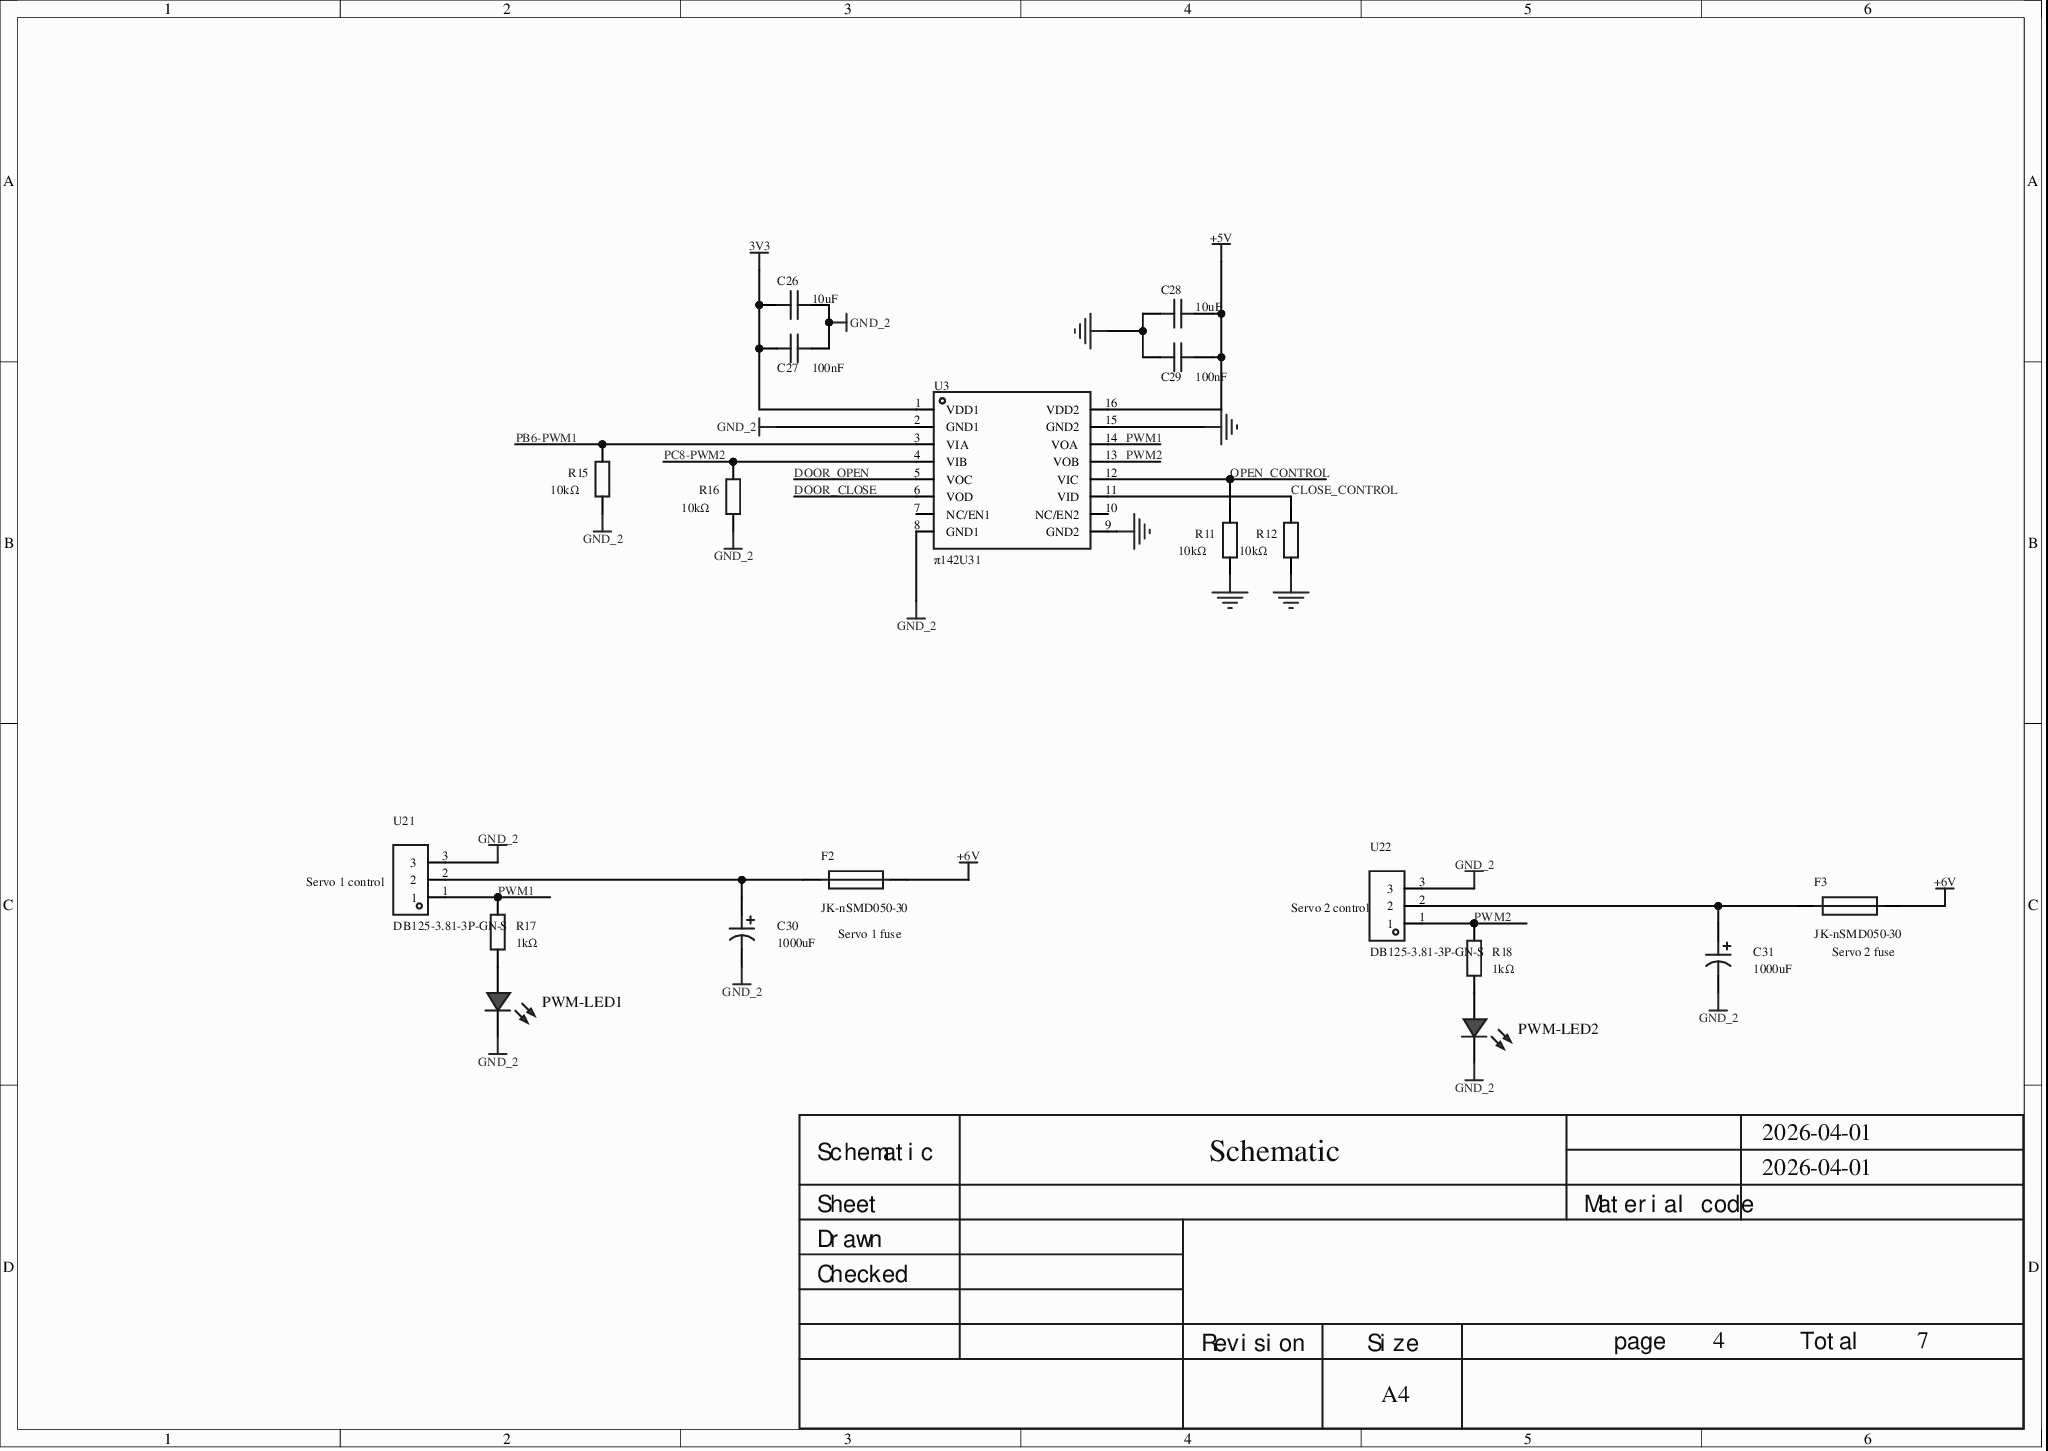
[diagram p0: MISC49876-5.schdoc]
# Altium project MISC49876-2.PrjPcb (part 2 of 2)
## Sheet MISC49876-5.schdoc (continued)
### Nets (continued)
CLOSE_CONTROL: R12.2 U3.11(VID)
DOOR_CLOSE: U3.6(VOD)
DOOR_OPEN: U3.5(VOC)
OPEN_CONTROL: R11.2 U3.12(VIC)
PB6-PWM1: R15.2 U3.3(VIA)
PC8-PWM2: R16.2 U3.4(VIB)
PWM1: R17.2 U3.14(VOA) U21.1
PWM2: R18.2 U3.13(VOB) U22.1
NetC30_1: C30.1 F2.1 U21.2
NetC31_1: C31.1 F3.1 U22.2
NetPWM-LED1_2: PWM-LED1.2(A) R17.1
NetPWM-LED2_2: PWM-LED2.2(A) R18.1

Not connected (* = marked no-connect by the designer): U3 7(NC/EN1) 10(NC/EN2)

### Notes on the sheet
- (near U21) Servo 1 control
- (near F2) Servo 1 fuse
- (near U22) Servo 2 control
- (near F3) Servo 2 fuse
- 2026-04-01
- Schematic
- Sheet
- Material code
- Checked
- Drawn
- Revision
- Size
- A4
- page
- 4
- Total
- 7

### Library data of the parts
C26 = GRM21BR61H106KE43L: Capacitance: 10uF; tolerance: ±10%; rated voltage: 50V; dielectric (temp. coefficient): X5R;; Manufacturer: muRata(村田); 3D Model: 1ba041120af144c991958decab20d241; 3D Model Transform: 78.74,51.181,0,0,0,0,0,0.0005,0; AddInBom: yes; ModelName: C0805_L2.0-W1.3-H1.3; Symbol: GRM21BR61H106KE43L; Device: GRM21BR61H106KE43L; LCSC Part Name: 10uF ±10% 50V; Supplier Footprint: 0805; Datasheet: https://atta.szlcsc.com/upload/public/pdf/source/20230811/95AAE0C9AF55EDC31B7A4D8B733F534E.pdf; Tolerance: ±10%; Voltage Rated: 50V; Temperature Coefficient: X5R; Supplier: LCSC; Supplier Part: C440198; Manufacturer Part: GRM21BR61H106KE43L; Value: 10uF; JLCPCB Part Class: Basic Part; ConvertToPcb: yes; FootprintName: C0805
C27 = CC0603KRX7R9BB104: Capacitance: 100nF; tolerance: ±10%; rated voltage: 50V; dielectric (temp. coefficient): X7R;; Manufacturer: YAGEO(国巨); Symbol: 0.1u; Add into BOM: yes; 3D Model: ac125912035d415993ca9572d50418b1; 3D Model Transform: 62.992,31.496,0,0,0,0,0,0,0; ModelName: C0603_L1.6-W0.8-H0.8; Device: CC0603KRX7R9BB104; Convert to PCB: yes; Origin Footprint: C0603; Supplier Part: C14663; Supplier: LCSC; Manufacturer Part: CC0603KRX7R9BB104; JLCPCB Part Class: Basic Part; LCSC Part Name: 100nF ±10% 50V; Supplier Footprint: 0603; Datasheet: https://atta.szlcsc.com/upload/public/pdf/source/20180910/C282072_33301C7F631E79921B82A8DAC6BCC5B3.pdf; Value: 100nF; Tolerance: ±10%; Voltage Rated: 50V; Temperature Coefficient: X7R; FootprintName: C0603
C28 = GRM21BR61H106KE43L: Capacitance: 10uF; tolerance: ±10%; rated voltage: 50V; dielectric (temp. coefficient): X5R;; Manufacturer: muRata(村田); AddInBom: yes; ModelId: 1ba041120af144c991958decab20d241; ModelName: C0805_L2.0-W1.3-H1.3; ModelTransform: 78.74,51.181,0,0,0,0,0,0.0005,0; Symbol: GRM21BR61H106KE43L; Device: GRM21BR61H106KE43L; Supplier: LCSC; Supplier Part: C440198; Manufacturer Part: GRM21BR61H106KE43L; Value: 10uF; JLCPCB Part Class: Basic Part; LCSC Part Name: 10uF ±10% 50V; Supplier Footprint: 0805; Datasheet: https://atta.szlcsc.com/upload/public/pdf/source/20230811/95AAE0C9AF55EDC31B7A4D8B733F534E.pdf; ConvertToPcb: yes; FootprintName: C0805; Tolerance: ±10%; Voltage Rated: 50V; Temperature Coefficient: X5R
C29 = CC0603KRX7R9BB104: as C6 on sheet MISC49876-3; Origin Footprint: C0603; Device: CC0603KRX7R9BB104; Supplier Part: C14663; Supplier: LCSC; Manufacturer Part: CC0603KRX7R9BB104; Add into BOM: yes; JLCPCB Part Class: Basic Part; LCSC Part Name: 100nF ±10% 50V; Supplier Footprint: 0603; Datasheet: https://atta.szlcsc.com/upload/public/pdf/source/20180910/C282072_33301C7F631E79921B82A8DAC6BCC5B3.pdf; FootprintName: C0603; Value: 100nF; Tolerance: ±10%; Voltage Rated: 50V; Temperature Coefficient: X7R
C30 C31 = SPZ0JM102E10C35RAXXX: Capacitance: 1000uF; tolerance: ±20%; rated voltage: 6.3V;; Manufacturer: AISHI(艾华集团); AddInBom: yes; ModelId: 983aa343eddc42b59ebb10541a88166e; ModelTransform: 247.99486,248.229,0,90,0,0,0,0,-196.85; Symbol: SPZ0JM102E10C35RAXXX; Device: SPZ0JM102E10C35RAXXX; LCSC Part Name: 1000uF ±20% 6.3V; SupplierPart: C5349927; ManufacturerPart: SPZ0JM102E10C35RAXXX; Supplier Footprint: 插件,D6.3xL10mm; JLCPCB Part Class: Extended Part; Datasheet: https://atta.szlcsc.com/upload/public/pdf/source/20230106/1004933EB9CF55C39AD0630773DFF44F.pdf; Supplier: LCSC; ConvertToPcb: yes; FootprintName: CAP-TH_BD6.3-P2.50-D0.5-FD; ModelName: CAP-TH_BD6.3-P2.50-D0.5-FD; Value: 1000uF; Tolerance: ±20%; Rated Voltage: 6.3V
F2 F3 = JK-nSMD050-30: Max voltage: 30V; max current: 100A; hold current: 500mA; trip current: 1A;; Manufacturer: JK(金科); Symbol: JK-NSMD050-30V; AddInBom: yes; ModelId: f1628daad26847a79b887277a2bc8541; ModelName: F1206_L3.2-W1.7-H0.6; ModelTransform: 125.984,66.929,0,0,0,0,0,0,0; Power Dissipation: 600mW; Resistance - Initial (Ri) (Min): 150mΩ; Resistance - Post Trip (R1) (Max): 300mΩ; Maximum Time to Trip: 100ms; Device: JK-nSMD050-30; Supplier: LCSC; Supplier Part: C720075; Manufacturer Part: JK-nSMD050-30; JLCPCB Part Class: Extended library; LCSC Part Name: 30V 500mA 1206自恢复; Supplier Footprint: 1206; Datasheet: https://atta.szlcsc.com/upload/public/pdf/source/20200810/C720075_06AF2D4541537091880CC35F0EFB49F8.pdf; ConvertToPcb: yes; FootprintName: F1206; Operating Voltage (Max): 30V; Current Rating (Max): 100A; Hold Current: 500mA; Trip Current: 1A; Operating Temperature: -40℃~+85℃
PWM-LED1 PWM-LED2 = LED_0603-R: Symbol: LED_R; Convert to PCB: yes; 3D Model: dd8257b0d61a4cd7b68939a056e08095; 3D Model Transform: 58.72,29.4,22.03,0,0,0,0,0,0; ModelName: LED-0603_R; Device: LED_0603-R; Add into BOM: yes; Supplier Footprint: 0603; FootprintName: LED_0603
R11 R12 R15 R16 = 0603WAF3301T5E: Resistor type: thick film resistor; resistance: 3.3kΩ; tolerance: ±1%; power: 100mW; max working voltage: 75V; temp. coefficient: ±100ppm/℃;; Manufacturer: UNI-ROYAL(厚声); 3D Model: fc143cca1e79419f9cd78b61e9279f08; 3D Model Transform: 31.8897,63.7794,0,90,0,0,0,0,0; AddInBom: yes; Symbol: 0603WAF3301T5E; Device: 0603WAF3301T5E; Value: 10kΩ; LCSC Part Name: 3.3kΩ ±1% 100mW 厚膜电阻; Supplier Footprint: 0603; Datasheet: https://atta.szlcsc.com/upload/public/pdf/source/20200306/C422600_1E6D84923E4A46A82E41ADD87F860B5C.pdf; Type: Thick film resistor; Tolerance: ±1%; Power(Watts): 100mW; Overload Voltage (Max): 75V; Temperature Coefficient: ±100ppm/℃; Operating Temperature Range: -55℃~+155℃; Supplier: LCSC; Manufacturer Part: 0603WAF3301T5E; JLCPCB Part Class: Basic library; ConvertToPcb: yes; FootprintName: R0603; ModelName: R0603
R17 R18 = 0603WAF1001T5E: Resistance: 1kΩ; tolerance: ±1%; power: 100mW; temp. coefficient: ±100ppm/℃; resistor type: thick film resistor;; Manufacturer: UNI-ROYAL(厚声); Symbol: 0603waf1301t5e; AddInBom: yes; ModelId: fc143cca1e79419f9cd78b61e9279f08; ModelTransform: 31.8897,63.7794,0,90,0,0,0,0,0; Overload Voltage (Max): 75V; Device: 0603WAF1001T5E; Supplier: LCSC; Manufacturer Part: 0603WAF1001T5E; Supplier Part: C21190; Value: 1kΩ; JLCPCB Part Class: Basic Part; LCSC Part Name: 1kΩ ±1% 100mW 厚膜电阻; Supplier Footprint: 0603; Datasheet: https://atta.szlcsc.com/upload/public/pdf/source/20200306/C422600_1E6D84923E4A46A82E41ADD87F860B5C.pdf; ConvertToPcb: yes; FootprintName: R0603; ModelName: R0603; Tolerance: ±1%; Power(Watts): 100mW; Temperature Coefficient: ±100ppm/℃; Type: Thick film resistor; Operating Temperature Range: -55℃~+155℃
U3 = π142U31: 通过使用成熟的标准半导体CMOS技术和iDivider技术，这些隔离组件提供了出色的性能特性和可靠性，优于光耦设备和其他集成隔离器等替代产品。智能分压器技术（iDivider技术）是一种新一代数字隔离器技术，它利用电容分压器原理直接跨隔离器电容传输电压信号，无需信号调制和解调。隔离器数据通道独立，有多种配置可供选择，耐压额定值为1.5kV rms至6.0kV rms，数据速率从直流到600Mbps。设备两侧的电源电压范围为3.0V至5.5V，可与低电压系统兼容，并能在隔离屏障上实现电压转换功能。当未施加输; Manufacturer: 2Pai Semi(荣湃); AddInBom: yes; ModelId: c21ec766ec2643efb3352f8441994f4e0819f05c4eef4c71ace90d822a990e87; ModelName: SOIC-16_L9.9-W3.9-H1.8-LS6.0-P1.27; ModelTransform: 389.763,236.454,0,0,0,0,0,0,0; Number of Forward Channels: 2; Data Rate(Max): 150Kbps; Isolation Voltage(Vrms): 3000; CMTI(kV/us): 150kV/us; Propagation Delay(tpd): 4.5us; Voltage - Supply(VCCA): 3V~5.5V; Symbol: π142U31; Device: π142U31; LCSC Part Name: 增强ESD 3.0 kVrms/6.0 kVrms 150Kbps四通道数字隔离器; SupplierPart: C471603; ManufacturerPart: π142U31; Supplier Footprint: SOIC-16; JLCPCB Part Class: Extended Part; Datasheet: https://item.szlcsc.com/datasheet/%25CF%2580142U31/478045.html; Supplier: LCSC; ConvertToPcb: yes; FootprintName: SOIC-16_L9.9-W3.9-P1.27-LS6.0-BL; Number of Reverse Channels: 2; Default Output: -; Features: Multi-voltage-domain interface; fail-safe output; Voltage - Supply(VCCB): 3V~5.5V; Operating Temperature: -40℃~+125℃
U21 U22 = DB125-3.81-3P-GN-S: 结构:1x3P;间距:3.81mm;颜色:绿色;安装方式:直插;额定电流:10A;额定电压:300V;排数:1;线规 - AWG:16~26;线规 - 平方毫米:0.5~1;每排PIN数:3;工作温度范围:-40℃~+105℃;; Manufacturer: DORABO(地博电气); AddInBom: yes; ModelId: eb9d9db6d88745c4b1f598d16985b52f; ModelName: CONN-TH_DB3.81-LI-3P-125; ModelTransform: 469.6739,291.338,0,0,0,0,-11.811,11.811,-157.48; Structure: 1x3P; Pitch: 3.81mm; Current Rating (Max): 10A; Voltage Rating (Max): 300V; Wire Gauge - AWG: 16~26; Wire Gauge - mm2: 0.5~1; Number of PINs Per Row: 3; Symbol: DB125-3.81-3P; Device: DB125-3.81-3P-GN-S; LCSC Part Name: 3.81mm 1x3P 排数:1 每排P数:3 直插; SupplierPart: C395879; ManufacturerPart: DB125-3.81-3P-GN-S; Supplier Footprint: 插件,P=3.81mm; JLCPCB Part Class: Extended library; Datasheet: https://atta.szlcsc.com/upload/public/pdf/source/20220823/CB89165D0F406880B925A92BEEA3FB50.pdf; Supplier: LCSC; ConvertToPcb: yes; FootprintName: CONN-TH_3P-P3.81_L7.4-W11.4; Color: Green; Mounting Style: Through-hole; Number of Pins: 3P; Number of Rows: 1; Operating Temperature Range: -40℃~+105℃

## Sheet MISC49876-4.schdoc
size 297 x 210 mm; Version: V1.0; @Project Name: MISC49876; @Page Count: 7; @Update Date: 2026-04-01; @Create Date: 2026-04-01; @Schematic Name: MISC49876; @Page No: 1; @Board Name: MISC49876; @Create Time: 07:49:54; @Update Time: 15:55:16
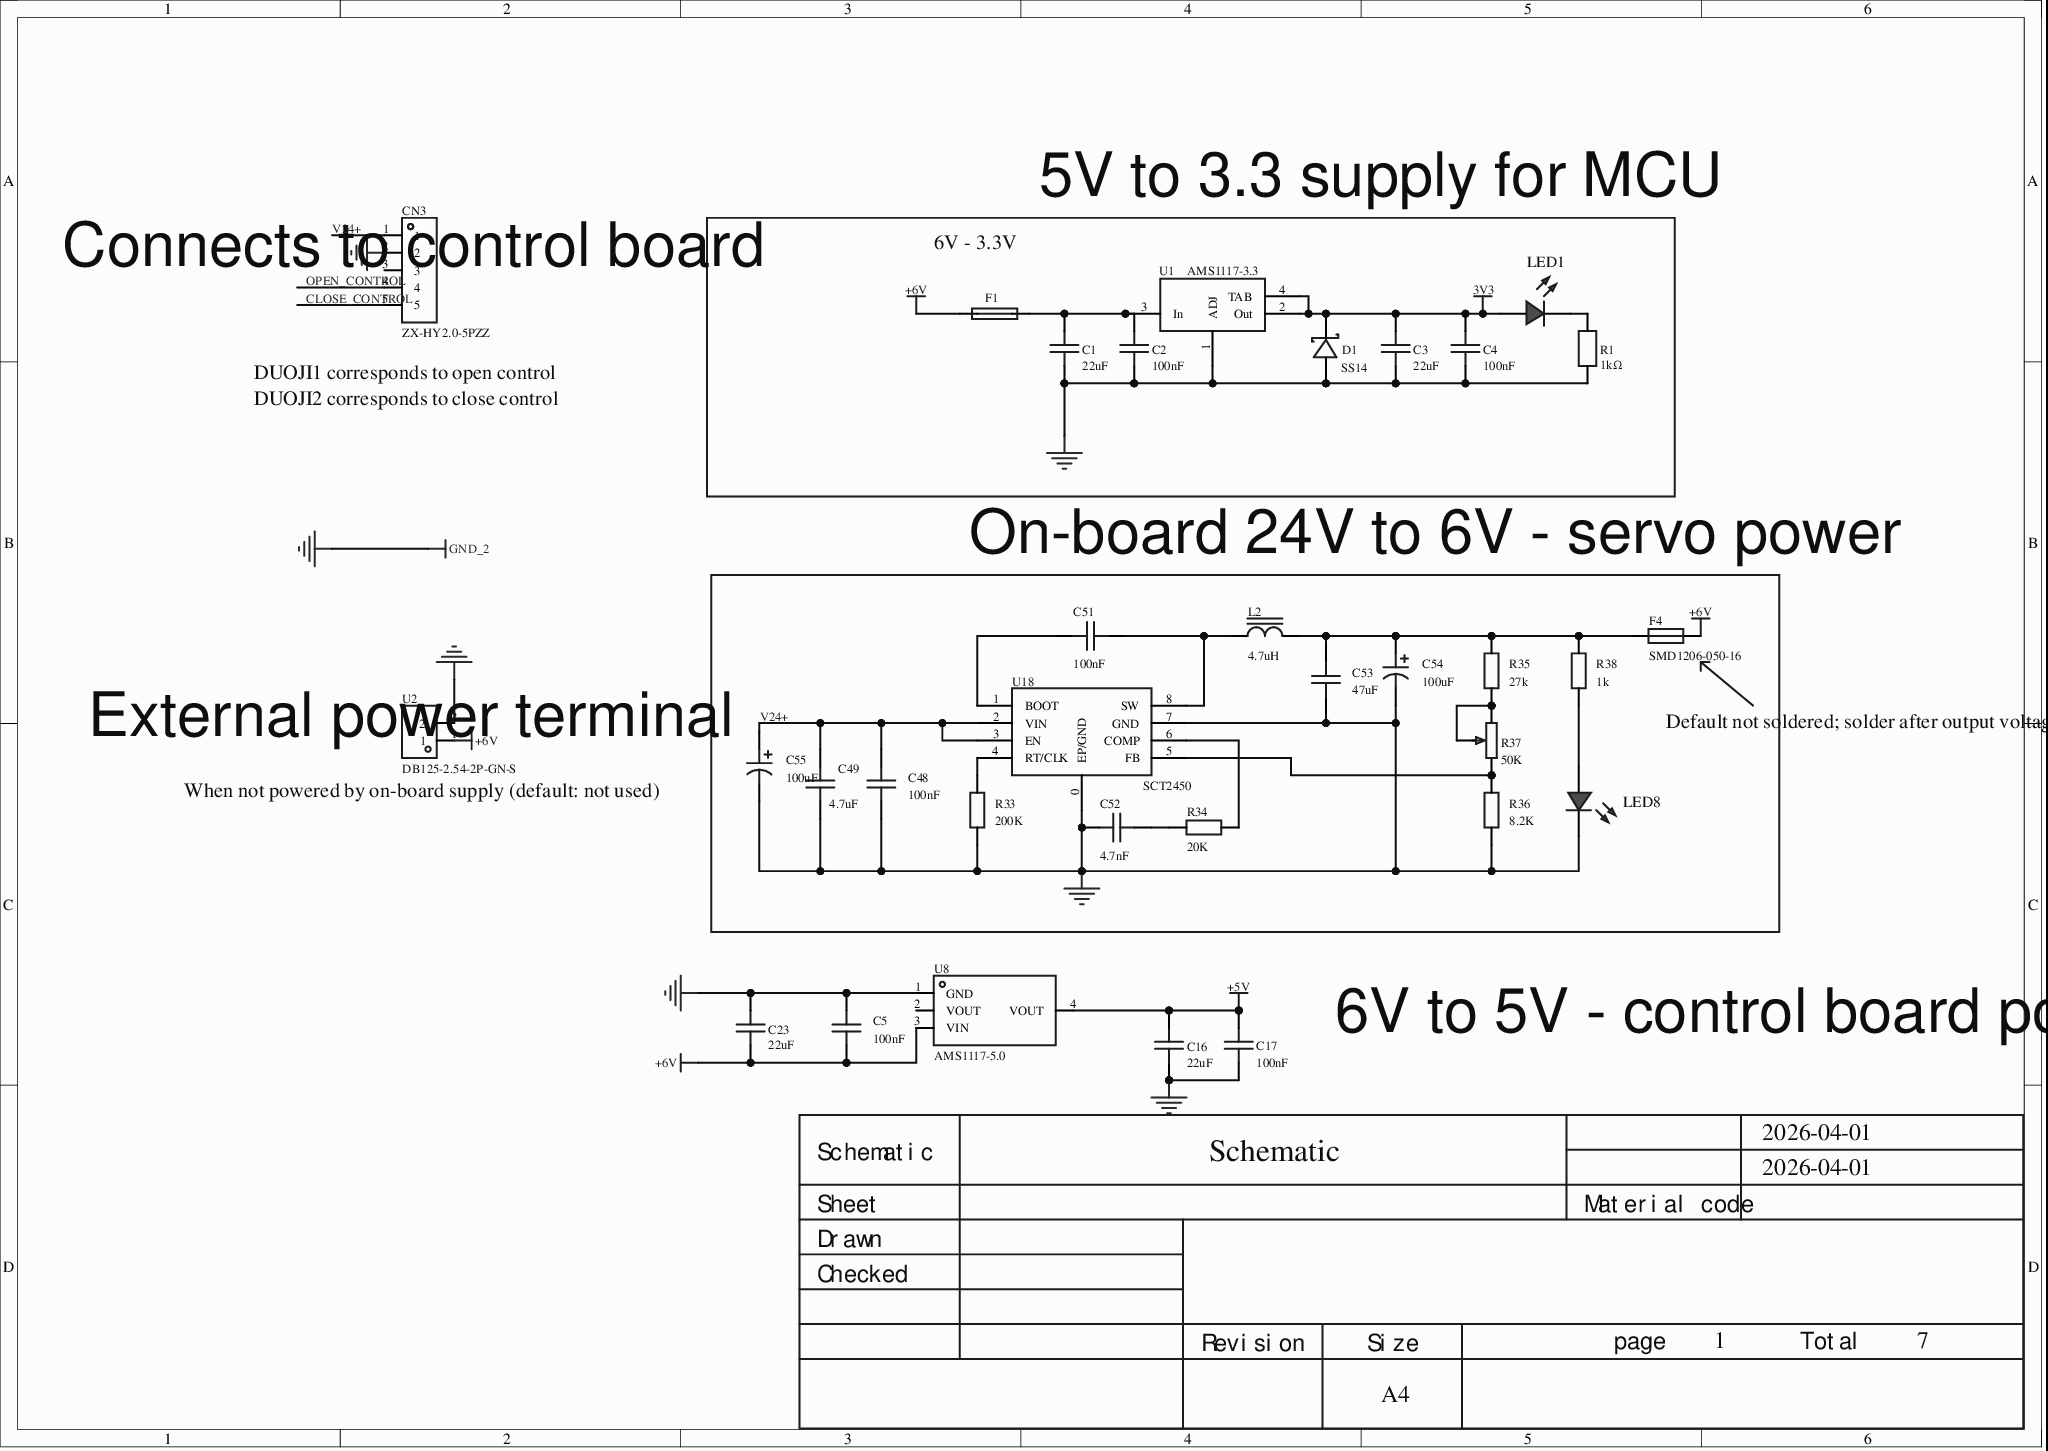
[diagram p1: MISC49876-4.schdoc]

### Parts
C1  22uF  [C0603]
C2  100nF  [C0603]
C3  22uF  [C0603]
C4  100nF  [C0603]
C5  100nF  [C0603]
C16  22uF  [C0603]
C17  100nF  [C0603]
C23  22uF  [C0603]
C48  100nF  [C0603]
C49  4.7uF  [C0603]
C51  100nF  [C0603]
C52  4.7nF  [C0603]
C53  47uF  [C0603]
C54  100uF  [CAP-TH_BD5.0-P2.00-D0.5-FD]
C55  100uF  [CAP-TH_BD5.0-P2.00-D0.5-FD]
CN3  ZX-HY2.0-5PZZ  [CONN-TH_5P-P2.00_ZX-HY2.0-5PZZ]
D1  SS14  [SMA_L4.2-W2.6-LS5.3-RD]
F1  PICOSMDC050S-2  [F0805]  (value not drawn)
F4  SMD1206-050-16  [F1206]
L2  4.7uH  [0630 TPC 7*7*3]
LED1  (no value)  [LED_0603]
LED8  (no value)  [LED_0603]
R1  1kΩ  [R0603]
R33  200K  [R0603]
R34  20K  [R0603]
R35  27k  [R0603]
R36  8.2K  [R0603]
R37  50K  [RESPOT3296]
R38  1k  [R0603]
U1  AMS1117-3.3  [SOT-223-3_L6.5-W3.4-P2.30-LS7.0-BR]
U2  DB125-2.54-2P-GN-S  [CONN-TH_DB125-2.54-2P-GN]
U8  AMS1117-5.0  [SOT-223_L6.5-W3.5-P2.30-LS7.0-BR]
U18  SCT2450  [SOP-8E]

### Blocks framed on the sheet
5V to 3.3 supply for MCU: C1-C4 D1 F1 LED1 R1 U1
On-board 24V to 6V - servo power: C48 C49 C51-C55 F4 L2 LED8 R33-R38 U18

### Nets
3V3: C3.2 C4.2 D1.1(C) LED1.2(A) U1.2(Out) U1.4(TAB)
+5V: C16.2 C17.2 U8.4(VOUT)
+6V: C5.1 C23.1 F1.1 F4.2 U2.1 U8.3(VIN)
GND_2: C1.1 C2.1 C3.1 C4.1 C5.2 C16.1 C17.1 C23.2 C48.1 C49.1 C52.2 C53.2 C54.2 C55.2 CN3.2 D1.2(A) LED8.1(C) R1.1 R33.1 R36.1 U1.1(ADJ) U2.2 U8.1(GND) U18.0(EP/GND) U18.7(GND)  [also labelled GND]
CLOSE_CONTROL: CN3.5
OPEN_CONTROL: CN3.4
V24+: C48.2 C49.2 C55.1 CN3.1 U18.2(VIN) U18.3(EN)
NetC1_2: C1.2 C2.2 F1.2 U1.3(In)
NetC51_1: C51.1 L2.1 U18.8(SW)
NetC51_2: C51.2 U18.1(BOOT)
NetC52_1: C52.1 R34.2
NetC53_1: C53.1 C54.1 F4.1 L2.2 R35.2 R38.2
NetLED1_1: LED1.1(C) R1.2
NetLED8_2: LED8.2(A) R38.1
NetR33_2: R33.2 U18.4(RT/CLK)
NetR34_1: R34.1 U18.6(COMP)
NetR35_1: R35.1 R37.1(TOP) R37.ADJ
NetR36_2: R36.2 R37.2(BOT) U18.5(FB)

Not connected (* = marked no-connect by the designer): CN3 3*; U8 2(VOUT)

### Notes on the sheet
- 6V - 3.3V
- (near CN3) Connects to control board
- (near CN3) DUOJI1 corresponds to open control
- DUOJI2 corresponds to close control
- External power terminal
- Default not soldered; solder after output voltage is adjusted
- (near C55) When not powered by on-board supply (default: not used)
- 6V to 5V - control board power match
- 2026-04-01
- Schematic
- Sheet
- Material code
- Checked
- Drawn
- Revision
- Size
- A4
- page
- 1
- Total
- 7

### Library data of the parts
C1 C3 = CL10A226MQ8NRNC: Capacitance: 22uF; tolerance: ±20%; rated voltage: 6.3V; dielectric (temp. coefficient): X5R;; Manufacturer: SAMSUNG(三星); Origin Footprint: C0805; Convert to PCB: yes; ModelId: ac125912035d415993ca9572d50418b1; ModelName: C0603_L1.6-W0.8-H0.8; ModelTransform: 62.992,31.496,0,0,0,0,0,0,0; Device: CL10A226MQ8NRNC; Symbol: 22uf; Supplier Part: C59461; Supplier: LCSC; Manufacturer Part: CL10A226MQ8NRNC; Add into BOM: yes; LCSC Part Name: 22uF ±20% 6.3V; Supplier Footprint: 0603; JLCPCB Part Class: Basic Part; Datasheet: https://atta.szlcsc.com/upload/public/pdf/source/20160218/1457707763339.pdf; FootprintName: C0603; Value: 22uF; Tolerance: ±20%; Voltage Rated: 6.3V; Temperature Coefficient: X5R
C2 C4 = CC0603KRX7R9BB104: Capacitance: 100nF; tolerance: ±10%; rated voltage: 50V; dielectric (temp. coefficient): X7R;; Manufacturer: YAGEO(国巨); Symbol: 0.1uf; Convert to PCB: yes; ModelId: ac125912035d415993ca9572d50418b1; ModelName: C0603_L1.6-W0.8-H0.8; ModelTransform: 62.992,31.496,0,0,0,0,0,0,0; Origin Footprint: C0603; Device: CC0603KRX7R9BB104; Supplier Part: C14663; Supplier: LCSC; Manufacturer Part: CC0603KRX7R9BB104; Add into BOM: yes; JLCPCB Part Class: Basic Part; LCSC Part Name: 100nF ±10% 50V; Supplier Footprint: 0603; Datasheet: https://atta.szlcsc.com/upload/public/pdf/source/20180910/C282072_33301C7F631E79921B82A8DAC6BCC5B3.pdf; FootprintName: C0603; Value: 100nF; Tolerance: ±10%; Voltage Rated: 50V; Temperature Coefficient: X7R
C5 = CAP_0603: Symbol: CapAcitance; 3D Model: ac125912035d415993ca9572d50418b1; 3D Model Transform: 62.992,31.496,0,0,0,0,0,0,0; ConvertToPcb: yes; ModelName: C0603_L1.6-W0.8-H0.8; Device: CAP_0603; Supplier Footprint: 0603; Value: 100nF; AddInBom: yes; FootprintName: C0603
C16 C23 = CL10A226MQ8NRNC: Capacitance: 22uF; tolerance: ±20%; rated voltage: 6.3V; dielectric (temp. coefficient): X5R;; Manufacturer: SAMSUNG(三星); Add into BOM: yes; Origin Footprint: C0805; 3D Model: ac125912035d415993ca9572d50418b1; 3D Model Transform: 62.992,31.496,0,0,0,0,0,0,0; ModelName: C0603_L1.6-W0.8-H0.8; Symbol: 22uf; Device: CL10A226MQ8NRNC; Convert to PCB: yes; Supplier Part: C59461; Supplier: LCSC; Manufacturer Part: CL10A226MQ8NRNC; LCSC Part Name: 22uF ±20% 6.3V; Supplier Footprint: 0603; JLCPCB Part Class: Basic Part; Datasheet: https://atta.szlcsc.com/upload/public/pdf/source/20160218/1457707763339.pdf; Value: 22uF; Tolerance: ±20%; Voltage Rated: 6.3V; Temperature Coefficient: X5R; FootprintName: C0603
C17 = CC0603KRX7R9BB104: Capacitance: 100nF; tolerance: ±10%; rated voltage: 50V; dielectric (temp. coefficient): X7R;; Manufacturer: YAGEO(国巨); Symbol: 0.1uf; Add into BOM: yes; 3D Model: ac125912035d415993ca9572d50418b1; 3D Model Transform: 62.992,31.496,0,0,0,0,0,0,0; ModelName: C0603_L1.6-W0.8-H0.8; Device: CC0603KRX7R9BB104; Convert to PCB: yes; Origin Footprint: C0603; Supplier Part: C14663; Supplier: LCSC; Manufacturer Part: CC0603KRX7R9BB104; JLCPCB Part Class: Basic Part; LCSC Part Name: 100nF ±10% 50V; Supplier Footprint: 0603; Datasheet: https://atta.szlcsc.com/upload/public/pdf/source/20180910/C282072_33301C7F631E79921B82A8DAC6BCC5B3.pdf; Value: 100nF; Tolerance: ±10%; Voltage Rated: 50V; Temperature Coefficient: X7R; FootprintName: C0603
C48 C49 C51-C53 = CAP_0603: Symbol: CapAcitance; ConvertToPcb: yes; ModelId: ac125912035d415993ca9572d50418b1; ModelName: C0603_L1.6-W0.8-H0.8; ModelTransform: 62.992,31.496,0,0,0,0,0,0,0; Device: CAP_0603; AddInBom: yes; Supplier Footprint: 0603; FootprintName: C0603
  C48 C51: Value: 100nF
  C49: Value: 4.7uF
  C52: Value: 4.7nF
  C53: Value: 47uF
C54 C55 = 1010160507R00: Capacitance: 100uF; rated voltage: 16V;; Manufacturer: NJCON(永立); AddInBom: yes; ModelId: aba3b94bdab6406eb4f45c9c765c730e; ModelTransform: 196.85,196.517,0,0,0,0,0,0,-196.85; Device: 1010160507R00; Symbol: 1010160507R00; LCSC Part Name: 100uF16V; SupplierPart: C2887206; ManufacturerPart: 1010160507R00; Supplier Footprint: 插件,5x7mm; JLCPCB Part Class: Extended library; Datasheet: https://atta.szlcsc.com/upload/public/pdf/source/20210903/5EA6DA58B86483524406FCF8856B737F.pdf; Supplier: LCSC; ConvertToPcb: yes; FootprintName: CAP-TH_BD5.0-P2.00-D0.5-FD; ModelName: CAP-TH_BD5.0-P2.00-D0.5-FD; Value: 100uF; Rated Voltage: 16V
CN3 = ZX-HY2.0-5PZZ: 插针结构:1x5P;间距:2mm;安装方式:直插;参考系列:HY;总PIN数:5P;排数:1;每排PIN数:5;行距:-;额定电流:2A;触头材质:黄铜;触头镀层:锡;工作温度范围:-25℃~+85℃;; Manufacturer: Megastar(兆星); 3D Model: 2570e755802c405a8e29ee13311d8084; 3D Model Transform: 472.8337,200.787,0,0,0,0,0,-16.142,-133.858; Pins Structure: 1x5P; Pitch: 2mm; Reference Series: HY; Number of PINs Per Row: 5; Current Rating (Max): 2A; AddInBom: yes; Symbol: ZX-HY2.0-5PZZ; Device: ZX-HY2.0-5PZZ; LCSC Part Name: 1x5P 间距:2mm 直插 系列:HY; Supplier Part: C7429581; Manufacturer Part: ZX-HY2.0-5PZZ; Supplier Footprint: 插件,P=2mm; JLCPCB Part Class: Extended library; Datasheet: https://atta.szlcsc.com/upload/public/pdf/source/20230619/C585B37C11F40AB39860A001D2C42AFA.pdf; Supplier: LCSC; Mounting Style: Through-hole; Number of Pins: 5P; Number of Rows: 1; Row Spacing: -; Contact Material: Brass; Contact Plating: Tin; Operating Temperature Range: -25℃~+85℃; ConvertToPcb: yes; FootprintName: CONN-TH_5P-P2.00_ZX-HY2.0-5PZZ; ModelName: CONN-TH_5P-P2.00_ZX-HY2.0-5PZZ
D1 = SS14_C2480: Diode configuration: single; forward voltage (Vf): 550mV@1A; DC reverse voltage (Vr): 40V; average rectified current (Io): 1A;; Manufacturer: MDD; Origin Footprint: SMA_L4.4-W2.8-LS5.4-RD; Convert to PCB: yes; ModelId: c9e8185d46a94015b9fa58a531b156cf; ModelTransform: 204.83943,103.346,0,0,0,0,-0.001,0.001,0; Reverse Leakage Current (Ir): 500uA@40V; Device: SS14_C2480; Symbol: ss14; Supplier: LCSC; Supplier Part: C2480; Manufacturer Part: SS14; Add into BOM: yes; LCSC Part Name: 电压:40V 电流:1A; Supplier Footprint: SMA(DO-214AC); JLCPCB Part Class: Basic Part; Datasheet: https://atta.szlcsc.com/upload/public/pdf/source/20230712/2DB6064CFBB99DE6DB116BEE8208BE66.pdf; FootprintName: SMA_L4.2-W2.6-LS5.3-RD; ModelName: SMA_L4.2-W2.6-LS5.3-RD; Diode Configuration: Single; Forward Voltage (Vf@If): 550mV@1A; Reverse Voltage (Vr): 40V; Average Rectified Current (Io): 1A
F1 = PICOSMDC050S-2: Max voltage: 6V; max current: 100A; hold current: 500mA; trip current: 1A;; Manufacturer: Littelfuse(美国力特); Convert to PCB: yes; ModelId: 57e2aa106f9143e8b6ab832aebb31c78; ModelName: F0805_L2.1-W1.4-H0.8; ModelTransform: 82.677,55.118,0,0,0,0,0.0005,0,0; Resistance - Initial (Ri) (Min): 800mΩ; Resistance - Post Trip (R1) (Max): 150mΩ; Maximum Time to Trip: 100ms; Origin Footprint: F0805; Device: PICOSMDC050S-2; Symbol: picosmdc050s-2; Supplier: LCSC; Supplier Part: C434721; Manufacturer Part: PICOSMDC050S-2; Add into BOM: yes; LCSC Part Name: 6V 500mA 0805自恢复 100毫秒内动作; Supplier Footprint: 0805; JLCPCB Part Class: Extended Part; Datasheet: https://atta.szlcsc.com/upload/public/pdf/source/20191009/C434721_930A0DCC097A55E27BDA9E3E8E5C1DDB.pdf; FootprintName: F0805; Operating Voltage (Max): 6V; Current Rating (Max): 100A; Hold Current: 500mA; Trip Current: 1A; Power Dissipation: -; Operating Temperature: -40℃~+85℃
F4 = SMD1206-050-16: Withstand voltage (Vmax): 16V; max current (Imax): 40A; hold current (Ihold): 500mA; trip current (Itrip): 1A;; Manufacturer: R+O(宏嘉诚); AddInBom: yes; ModelId: f1628daad26847a79b887277a2bc85410819f05c4eef4c71ace90d822a990e87; ModelName: F1206_L3.2-W1.7-H0.6; ModelTransform: 125.984,66.929,0,0,0,0,0,0,0; Power Dissipation: 600mW; Resistance - Initial (Ri) (Min): 150mΩ; Resistance - Post Trip (R1) (Max): 750mΩ; Time to Trip(Max): 100ms; Symbol: SMD1206-050-16; Device: SMD1206-050-16; LCSC Part Name: SMD1206-050-16; SupplierPart: C46641014; ManufacturerPart: SMD1206-050-16; Supplier Footprint: 1206; JLCPCB Part Class: Extended Part; Datasheet: https://item.szlcsc.com/datasheet/SMD1206-050-16/48798720.html; Supplier: LCSC; ConvertToPcb: yes; FootprintName: F1206; Voltage - Max: 16V; Current - Max: 40A; Hold Current: 500mA; Trip Current: 1A; Operating Temperature: -40℃~+85℃; Length: 3.6mm; Width: 1.9mm; Height: 0.8mm
L2 = Ind-Power: AddInBom: yes; DCR: .5m; Imax: 5A; Origin Footprint 2: CD31; Origin Footprint 3: CD32; Origin Footprint 4: CD42; Origin Footprint 5: CD43; Origin Footprint 6: CD52; Origin Footprint 7: CD53; Origin Footprint 8: CD54; Origin Footprint 9: CD73; Origin Footprint 10: CD75; Origin Footprint 11: CD104; Origin Footprint 12: CD105; Origin Footprint 13: CD106; Origin Footprint 14: 127 Shielded 12.5*12.5*7; Origin Footprint 15: 1050 TPC 10*10*5; Origin Footprint 16: 1265 TPC 12*12*6.5; Origin Footprint 17: CD104R; Origin Footprint 18: SLO2520; Origin Footprint 19: 1365 TPC 13*13*6.5; Origin Footprint 20: INDUCTOR; Origin Footprint 21: 0402 TPC 4*4*2; Symbol: Ind-Power; Device: Ind-Power; ConvertToPcb: yes; Published: 8-Jun-2000; Revision: July-2002: Re-released for DXP Platform.; Price(RMB): 0.000; Value: 4.7uH; FootprintName: 0630 TPC 7*7*3; Publisher: Altium Limited
LED1 LED8 = LED_0603-R: as PWM-LED1 on sheet MISC49876-5; Device: LED_0603-R; Add into BOM: yes; Supplier Footprint: 0603; FootprintName: LED_0603
R1 = 0603WAF1001T5E: Resistance: 1kΩ; tolerance: ±1%; power: 100mW; temp. coefficient: ±100ppm/℃; resistor type: thick film resistor;; Manufacturer: UNI-ROYAL(厚声); Symbol: 1k; Convert to PCB: yes; ModelId: fc143cca1e79419f9cd78b61e9279f08; ModelTransform: 31.8897,63.7794,0,90,0,0,0,0,0; Overload Voltage (Max): 75V; Origin Footprint: R0603; Device: 0603WAF1001T5E; Supplier Part: C21190; Supplier: LCSC; Manufacturer Part: 0603WAF1001T5E; Add into BOM: yes; LCSC Part Name: 1kΩ ±1% 100mW 厚膜电阻; Supplier Footprint: 0603; JLCPCB Part Class: Basic Part; Datasheet: https://atta.szlcsc.com/upload/public/pdf/source/20200306/C422600_1E6D84923E4A46A82E41ADD87F860B5C.pdf; FootprintName: R0603; ModelName: R0603; Value: 1kΩ; Tolerance: ±1%; Power(Watts): 100mW; Temperature Coefficient: ±100ppm/℃; Type: Thick film resistor; Operating Temperature Range: -55℃~+155℃
R33-R36 R38 = Res_0603: Symbol: Resistor; ConvertToPcb: yes; ModelId: fc143cca1e79419f9cd78b61e9279f08; ModelTransform: 31.8897,63.7794,0,90,0,0,0,0,0; Device: Res_0603; AddInBom: yes; Supplier Footprint: 0603; FootprintName: R0603; ModelName: R0603
  R33: Value: 200K
  R34: Value: 20K
  R35: Value: 27k
  R36: Value: 8.2K
  R38: Value: 1k
R37 = Res-Adj-3p: AddInBom: yes; Value: 10K; Origin Footprint 2: RESPOTSMALL; Origin Footprint 3: EVM3-3x3ADJ; Origin Footprint 4: RESPOT3386P; Symbol: Res-Adj-3p; Device: Res-Adj-3p; ConvertToPcb: yes; FootprintName: RESPOT3296
U1 = AMS1117-3.3_C6186: Output type: fixed; max input voltage: -; output voltage: 3.3V; output current: 1A; PSRR: 72dB@(120Hz); output polarity: positive;; Manufacturer: AMS; Origin Footprint: SOT-223_L6.7-W3.5-P2.30-BR; Convert to PCB: yes; ModelId: 925194bf9823436183a3e0b978a8d076; ModelName: SOT-223-4P_L6.5-W3.5-H1.6-LS7.0-P2.30; ModelTransform: 279.89794,255.905,0,180,0,0,-3.9385,-0.0005,0; Dropout Voltage: 1.3V@(800mA); Number of Outputs: 1; Device: AMS1117-3.3_C6186; Symbol: ams1117; Supplier: LCSC; Manufacturer Part: AMS1117-3.3; image: C6188.jpg; Supplier Part: C6186; Add into BOM: yes; LCSC Part Name: 输出3.3V 1A; Supplier Footprint: SOT-223-3; JLCPCB Part Class: Basic Part; Datasheet: https://atta.szlcsc.com/upload/public/pdf/source/20180727/C6186_7A095716F0823C02F1997A905E26C086.pdf; FootprintName: SOT-223-3_L6.5-W3.4-P2.30-LS7.0-BR; Output Type: Fixed; Maximum Input Voltage: -; Output Voltage: 3.3V; Output Current: 1A; Power Supply Rejection Ratio (PSRR): 72dB@(120Hz); Quiescent Current (Ground Current): -; Noise: -; Feature: -; Operating Temperature: -; Output Polarity: Positive
U2 = DB125-2.54-2P-GN-S: 结构:1x2P;间距:2.54mm;颜色:绿色;安装方式:直插;排数:1;每排PIN数:2;额定电流:7A;额定电压:150V;线规 - AWG:18~26;线规 - 平方毫米:1;工作温度:-40℃~+105℃;; Manufacturer: DORABO(地博电气); AddInBom: yes; ModelId: e364713d301b433da8ecef6fca46e9720819f05c4eef4c71ace90d822a990e87; ModelTransform: 218.90114,248.031,0,0,0,0,0,-0.591,-137.795; Number of Positions or Pins: 1x2P; Pitch: 2.54mm; Number of PINs Per Row: 2; Current Rating: 7A; Voltage Rating (Max): 150V; Wire Gauge - AWG: 18~26; Wire Gauge - mm2: 1; Symbol: DB125-2.54-2P-GN; Device: DB125-2.54-2P-GN-S; LCSC Part Name: 1x2P 2.54mm 直插 排数:1 每排P数:2; SupplierPart: C918120; ManufacturerPart: DB125-2.54-2P-GN-S; Supplier Footprint: 插件,P=2.54mm; JLCPCB Part Class: Extended Part; Datasheet: https://item.szlcsc.com/datasheet/DB125-2.54-2P-GN-S/993699.html; Supplier: LCSC; ConvertToPcb: yes; FootprintName: CONN-TH_DB125-2.54-2P-GN; ModelName: CONN-TH_DB125-2.54-2P-GN; Color: Green; Mounting Type: Through-hole; Number of Pins: 2P; Number of Rows: 1; Operating Temperature: -40℃~+105℃
U8 = AMS1117-5.0_C6187: Output type: fixed; operating voltage: 15V; output voltage: 5V; output current: 1A; PSRR: 60dB; output polarity: positive;; Manufacturer: AMS; AddInBom: yes; ModelId: 925194bf9823436183a3e0b978a8d0760819f05c4eef4c71ace90d822a990e87; ModelName: SOT-223-4P_L6.5-W3.5-H1.6-LS7.0-P2.30; ModelTransform: 279.89794,255.905,0,180,0,0,0.0005,0.0005,0; Voltage Dropout: 1.3V; Number of Outputs: 1; Symbol: AMS1117-5.0; Device: AMS1117-5.0_C6187; LCSC Part Name: 输入15V 输出5V 1A; SupplierPart: C6187; ManufacturerPart: AMS1117-5.0; Supplier Footprint: SOT-223; JLCPCB Part Class: Basic Part; Datasheet: https://item.szlcsc.com/datasheet/AMS1117-5.0/6653.html; Supplier: LCSC; ConvertToPcb: yes; FootprintName: SOT-223_L6.5-W3.5-P2.30-LS7.0-BR; Output Type: Fixed; Voltage - Supply: 15V; Output Voltage: 5V; Output Current: 1A; Power Supply Rejection Ratio (PSRR): 60dB; standby current: -; Noise: -; Features: -; Operating Temperature: -40℃~+125℃; Output Configuration: Positive
U18 = SCT2450: AddInBom: yes; Symbol: SCT2450; Device: SCT2450; ConvertToPcb: yes; FootprintName: SOP-8E

## Nets that join several sheets
3V3: MISC49876-3 (25 pins), MISC49876-5 (C26.1 C27.2 U3.1), MISC49876-4 (6 pins)
+5V: MISC49876-5 (C28.2 C29.1 U3.16), MISC49876-4 (C16.2 C17.2 U8.4)
+6V: MISC49876-5 (F2.2 F3.2), MISC49876-4 (6 pins)
GND_2: MISC49876-3 (34 pins), MISC49876-5 (18 pins), MISC49876-4 (25 pins)
CLOSE_CONTROL: MISC49876-5 (R12.2 U3.11), MISC49876-4 (CN3.5)
DOOR_CLOSE: MISC49876-3 (U4.36), MISC49876-5 (U3.6)
DOOR_OPEN: MISC49876-3 (U4.35), MISC49876-5 (U3.5)
OPEN_CONTROL: MISC49876-5 (R11.2 U3.12), MISC49876-4 (CN3.4)
PB6-PWM1: MISC49876-3 (U4.58), MISC49876-5 (R15.2 U3.3)
PC8-PWM2: MISC49876-3 (U4.39), MISC49876-5 (R16.2 U3.4)